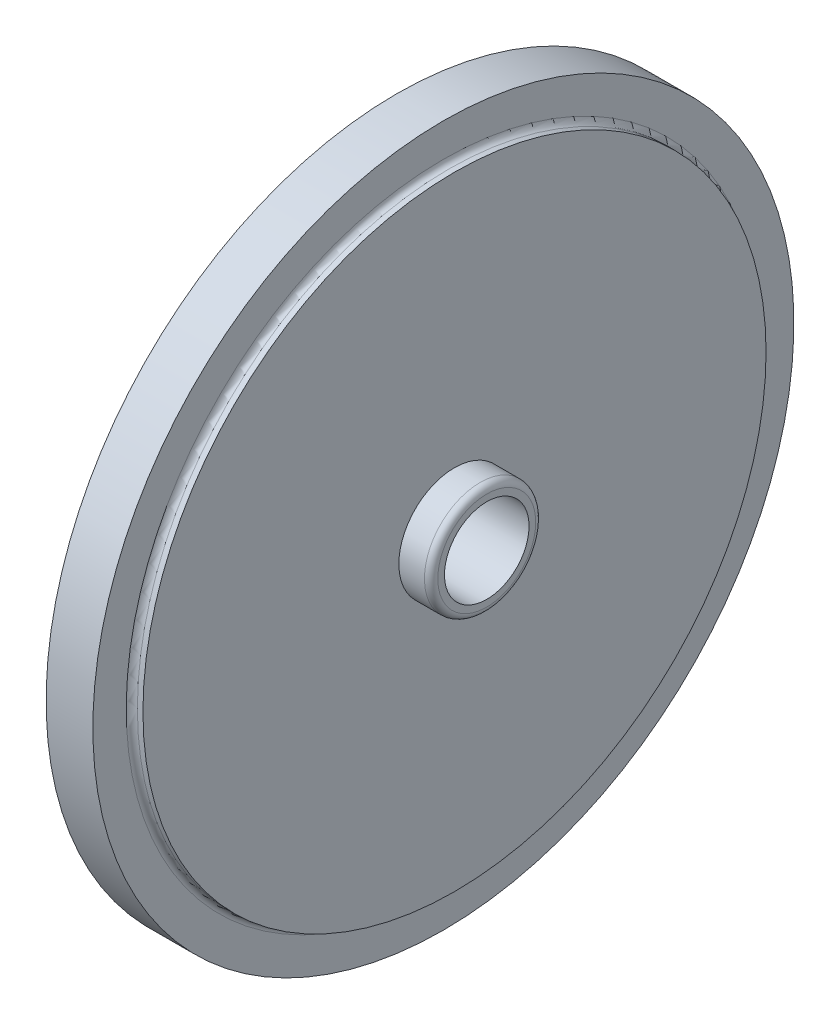
from build123d import *


with BuildPart() as part:
    # Sketch1 → Revolve1 (revolve)
    with BuildSketch(Plane.XY):
        with BuildLine():
            Line((-130.8, 157.5), (-151.8, 157.5))
            Line((-151.8, 157.5), (-151.8, 145.5))
            Line((-151.8, 145.5), (-151.8, 141.5))
            Line((-151.8, 141.5), (-150.8, 141.5))
            ThreePointArc((-150.8, 141.5), (-150.092893219, 141.207106781), (-149.8, 140.5))
            Line((-149.8, 140.5), (-149.8, 131.984995497))
            ThreePointArc((-149.8, 131.984995497), (-149.701421663, 131.552053256), (-149.425122031, 131.204468466))
            ThreePointArc((-149.425122031, 131.204468466), (-140.856955291, 120.42571931), (-137.8, 107))
            Line((-137.8, 107), (-137.8, 82.5))
            Line((-137.8, 82.5), (-137.8, 25))
            Line((-137.8, 25), (-144.3, 25))
            ThreePointArc((-144.3, 25), (-146.421320344, 24.121320344), (-147.3, 22))
            Line((-147.3, 22), (-147.3, 19))
            Line((-147.3, 19), (-111.3, 19))
            Line((-111.3, 19), (-111.3, 22))
            ThreePointArc((-111.3, 22), (-112.178679656, 24.121320344), (-114.3, 25))
            Line((-114.3, 25), (-125.8, 25))
            Line((-125.8, 25), (-125.8, 82.5))
            Line((-125.8, 82.5), (-125.8, 140))
            Line((-125.8, 140), (-128.3, 140))
            ThreePointArc((-128.3, 140), (-130.067766953, 140.732233047), (-130.8, 142.5))
            Line((-130.8, 142.5), (-130.8, 157.5))
        make_face()
    revolve(axis=Axis((-55, 0, 0), (-1, 0, 0)))


solid = part.part
